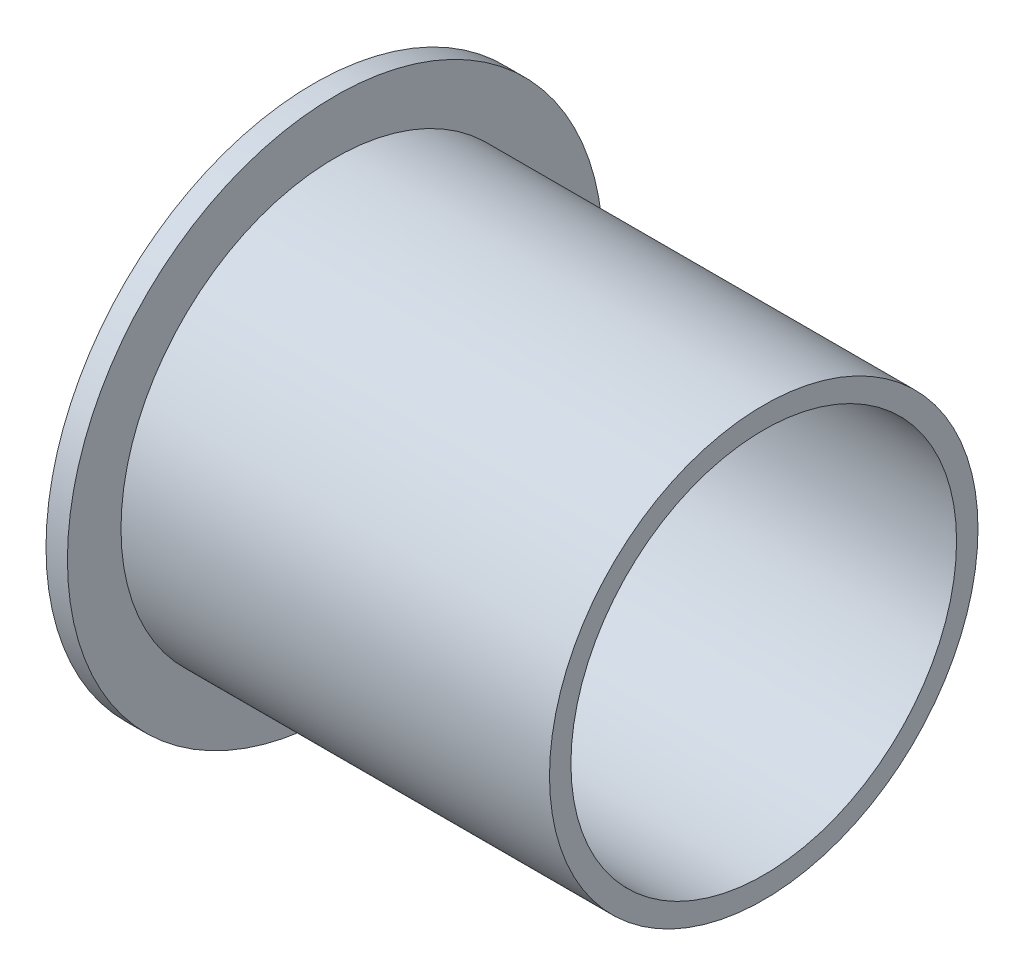
SolidWorks part; units mm, degrees
material "尼龙 101"
ref_plane "前视基准面" through (0, 0, 0) normal (0, 0, 1) x (1, 0, 0)
ref_plane "上视基准面" through (0, 0, 0) normal (0, 1, 0) x (1, 0, 0)
ref_plane "右视基准面" through (0, 0, 0) normal (1, 0, 0) x (0, 0, -1)
sketch "草图1" plane through (0, 0, 0) normal (0, 0, 1) x (1, 0, 0)
  line L0 (0, 30.304) -> (0, 0) construction
  line L1 (0, 0) -> (39.5369, 0) construction
  line L2 (0, 25) -> (2, 25)
  line L3 (2, 25) -> (2, 20)
  line L4 (2, 20) -> (42, 20)
  line L5 (42, 20) -> (42, 18)
  line L6 (42, 18) -> (2, 18)
  line L7 (2, 18) -> (2, 5)
  line L8 (2, 5) -> (0, 5)
  line L9 (0, 5) -> (0, 25)
  dimension "D1" = 10
  dimension "D2" = 40
  dimension "D3" = 2
  dimension "D4" = 2
  dimension "D5" = 5
  dimension "D6" = 40
revolve "旋转1" add sketch "草图1" angle 360 about L1
